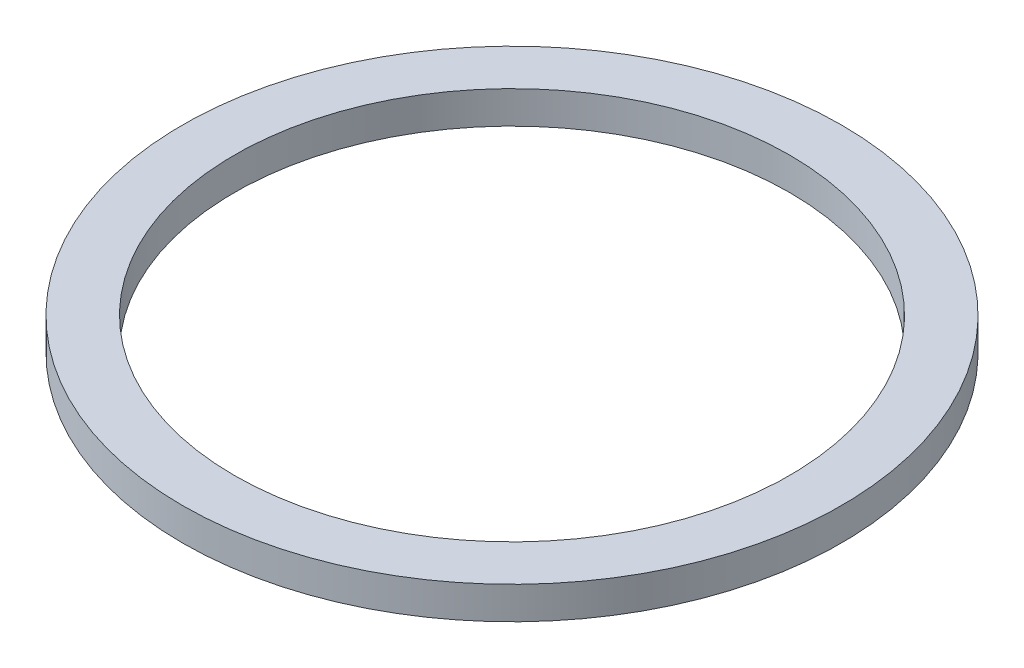
SolidWorks part; units mm, degrees
ref_plane "Front Plane" through (0, 0, 0) normal (0, 0, 1) x (1, 0, 0)
ref_plane "Top Plane" through (0, 0, 0) normal (0, 1, 0) x (1, 0, 0)
ref_plane "Right Plane" through (0, 0, 0) normal (1, 0, 0) x (0, 0, -1)
other "Configuration Table"
sketch "Sketch1" plane through (0, 0, 0) normal (0, 1, 0) x (1, 0, 0)
  circle A0 centre (0, 0) radius 23.5
  circle A1 centre (0, 0) radius 27.9
  dimension "D1" = 47
  dimension "D2" = 55.8
extrude "Boss-Extrude1" add sketch "Sketch1" along normal blind 2.75
